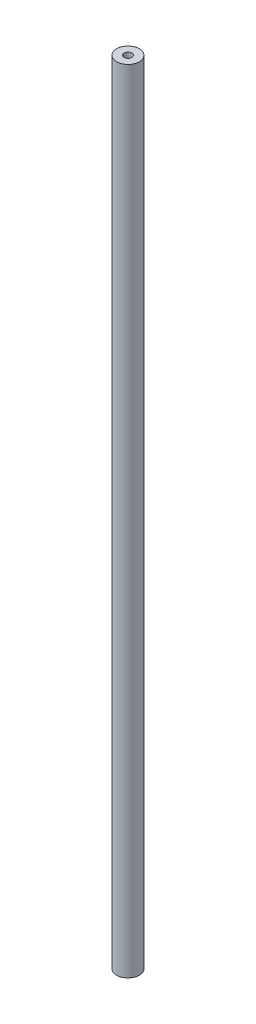
from build123d import *

# Parameters (mm, degrees)
SKETCH1_R             = 10
BOSS_EXTRUDE1_DEPTH   = 700
M8_TAPPED_HOLE1_D     = 6.8
M8_TAPPED_HOLE1_DEPTH = 19.75
M8_TAPPED_HOLE1_TIP   = 2.042926105
M8_TAPPED_HOLE2_D     = 6.8
M8_TAPPED_HOLE2_DEPTH = 19.75
M8_TAPPED_HOLE2_TIP   = 2.042926105


with BuildPart() as part:
    # Sketch1 → Boss-Extrude1 (new body)
    with BuildSketch(Plane(origin=(0, 0, 0), x_dir=(1, 0, 0), z_dir=(0, 1, 0))):
        with Locations(Location((0, 0, 0), (0, 0, 270))):
            Circle(SKETCH1_R)
    extrude(amount=BOSS_EXTRUDE1_DEPTH)

    # M8 Tapped Hole1
    with Locations(Plane(origin=(0, 700, 0), x_dir=(1, 0, 0), z_dir=(0, 1, 0))):
        with Locations((0, 0)):
            Hole(M8_TAPPED_HOLE1_D / 2, depth=M8_TAPPED_HOLE1_DEPTH)
            with Locations((0, 0, -(M8_TAPPED_HOLE1_DEPTH + M8_TAPPED_HOLE1_TIP / 2))):  # 118° drill point
                Cone(0, M8_TAPPED_HOLE1_D / 2, M8_TAPPED_HOLE1_TIP, mode=Mode.SUBTRACT)

    # M8 Tapped Hole2
    with Locations(Plane(origin=(0, 0, 0), x_dir=(-1, 0, 0), z_dir=(0, -1, 0))):
        with Locations((0, 0)):
            Hole(M8_TAPPED_HOLE2_D / 2, depth=M8_TAPPED_HOLE2_DEPTH)
            with Locations((0, 0, -(M8_TAPPED_HOLE2_DEPTH + M8_TAPPED_HOLE2_TIP / 2))):  # 118° drill point
                Cone(0, M8_TAPPED_HOLE2_D / 2, M8_TAPPED_HOLE2_TIP, mode=Mode.SUBTRACT)


solid = part.part
